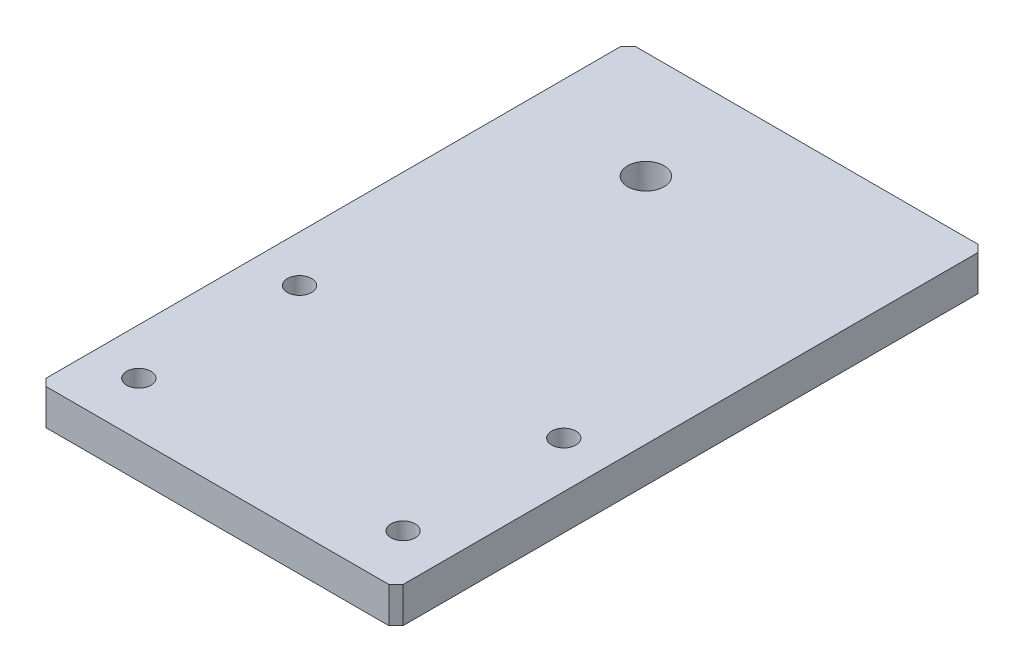
from build123d import *

# Parameters (mm, degrees)
SKETCH_1_W              = 100
SKETCH_1_H              = 165
EXTRUDE_1_DEPTH         = 10
CHAMFER_1_SIZE          = 2
HOLE_WIZARD_M12_1_D     = 10.2
HOLE_WIZARD_M12_1_DEPTH = 32.75
HOLE_WIZARD_M12_1_TIP   = 3.064389157
HOLE_WIZARD_M8_2_D      = 6.8
HOLE_WIZARD_M8_2_DEPTH  = 22.25
HOLE_WIZARD_M8_2_TIP    = 2.042926105


with BuildPart() as part:
    # 草图1 → 凸台-拉伸1 (new body)
    with BuildSketch(Plane(origin=(0, 0, 0), x_dir=(1, 0, 0), z_dir=(0, 1, 0))):
        with Locations((50, 82.5)):
            Rectangle(SKETCH_1_W, SKETCH_1_H)
    extrude(amount=EXTRUDE_1_DEPTH)

    # 倒角1
    chamfer_1_edges = [part.edges().sort_by_distance(p)[0] for p in [
        (0, 5, -165),
        (100, 5, -165),
        (100, 5, 0),
        (0, 5, 0),
    ]]
    chamfer(chamfer_1_edges, length=CHAMFER_1_SIZE)

    # M12 螺纹孔1
    with Locations(Plane(origin=(35, 10, -135), x_dir=(0, 0, 1), z_dir=(0, 1, 0))):
        with Locations((0, 0)):
            Hole(HOLE_WIZARD_M12_1_D / 2, depth=HOLE_WIZARD_M12_1_DEPTH)
            with Locations((0, 0, -(HOLE_WIZARD_M12_1_DEPTH + HOLE_WIZARD_M12_1_TIP / 2))):  # 118° drill point
                Cone(0, HOLE_WIZARD_M12_1_D / 2, HOLE_WIZARD_M12_1_TIP, mode=Mode.SUBTRACT)

    # M8 螺纹孔2
    with Locations(Plane(origin=(0, 10, 0), x_dir=(1, 0, 0), z_dir=(0, 1, 0))):
        with Locations((13, 60), (13, 15), (87, 15), (87, 60)):
            Hole(HOLE_WIZARD_M8_2_D / 2, depth=HOLE_WIZARD_M8_2_DEPTH)
            with Locations((0, 0, -(HOLE_WIZARD_M8_2_DEPTH + HOLE_WIZARD_M8_2_TIP / 2))):  # 118° drill point
                Cone(0, HOLE_WIZARD_M8_2_D / 2, HOLE_WIZARD_M8_2_TIP, mode=Mode.SUBTRACT)


solid = part.part
